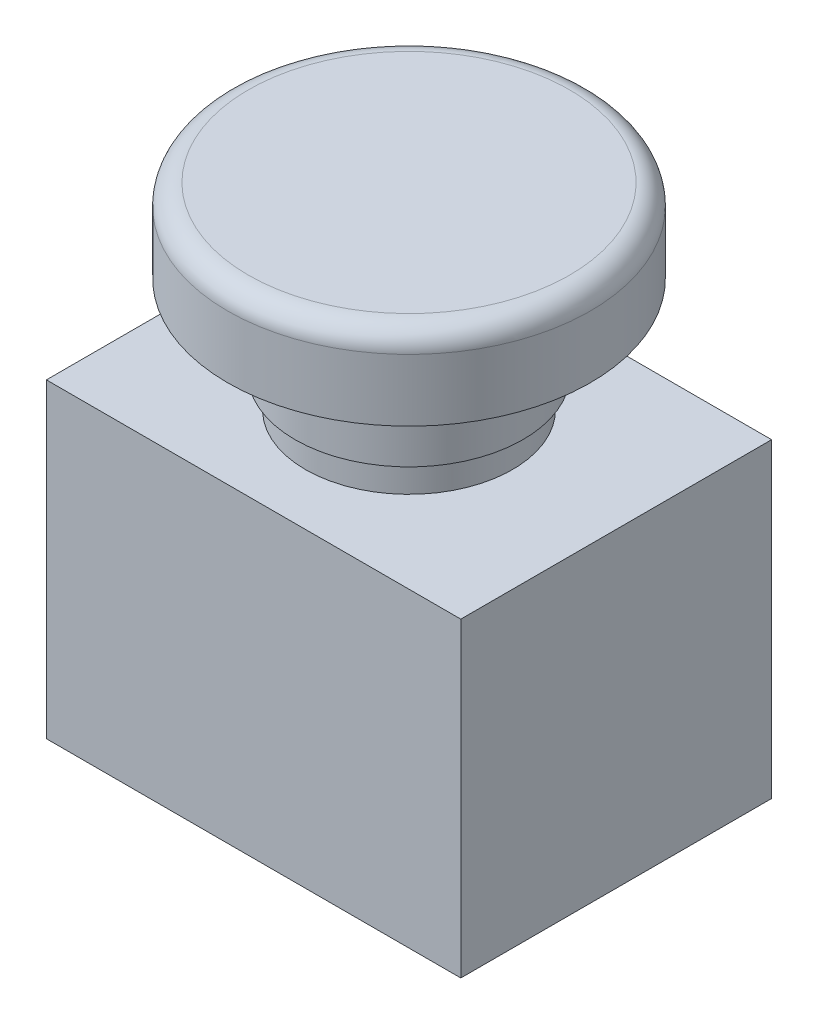
from build123d import *

# Parameters (mm, degrees)
SKETCH1_W          = 40
SKETCH1_H          = 30
EXTRUDE1_DEPTH     = 15
SKETCH2_R          = 11
EXTRUDE2_DEPTH     = 10
SKETCH3_R          = 10
EXTRUDE3_DEPTH     = 1
SKETCH4_R          = 17.5
EXTRUDE4_DEPTH     = 8
FILLET1_R          = 2
SKETCH5_OUTSIDE_W  = 56.458
SKETCH5_OUTSIDE_H  = 51.458
SKETCH5_OUTSIDE_R  = 10
CUT_EXTRUDE1_DEPTH = 3


with BuildPart() as part:
    # Sketch1 → Extrude1 (new, symmetric)
    with BuildSketch(Plane(origin=(0, 0, 0), x_dir=(1, 0, 0), z_dir=(0, 1, 0))):
        Rectangle(SKETCH1_W, SKETCH1_H)
    extrude(amount=EXTRUDE1_DEPTH, both=True)

    # Sketch2 → Extrude2 (add)
    with BuildSketch(Plane(origin=(0, 15, 0), x_dir=(1, 0, 0), z_dir=(0, 1, 0))):
        with Locations(Location((0, 0, 0), (0, 0, 270))):
            Circle(SKETCH2_R)
    extrude(amount=EXTRUDE2_DEPTH)

    # Sketch3 → Extrude3 (add)
    with BuildSketch(Plane(origin=(0, 25, 0), x_dir=(1, 0, 0), z_dir=(0, 1, 0))):
        with Locations(Location((0, 0, 0), (0, 0, 270))):
            Circle(SKETCH3_R)
    extrude(amount=EXTRUDE3_DEPTH)

    # Sketch4 → Extrude4 (add)
    with BuildSketch(Plane(origin=(0, 26, 0), x_dir=(1, 0, 0), z_dir=(0, 1, 0))):
        with Locations(Location((0, 0, 0), (0, 0, 270))):
            Circle(SKETCH4_R)
    extrude(amount=EXTRUDE4_DEPTH)

    # Fillet1
    fillet1_edges = [part.edges().sort_by_distance(p)[0] for p in [
        (0, 34, -17.5),
    ]]
    fillet(fillet1_edges, radius=FILLET1_R)

    # Sketch5 outside → Cut-Extrude1 (cut)
    with BuildSketch(Plane(origin=(0, 18, 0), x_dir=(-1, 0, 0), z_dir=(0, 1, 0))):
        Rectangle(SKETCH5_OUTSIDE_W, SKETCH5_OUTSIDE_H)
        with Locations(Location((0, 0, 0), (0, 0, 90))):
            Circle(SKETCH5_OUTSIDE_R, mode=Mode.SUBTRACT)
    extrude(amount=-CUT_EXTRUDE1_DEPTH, mode=Mode.SUBTRACT)


solid = part.part
